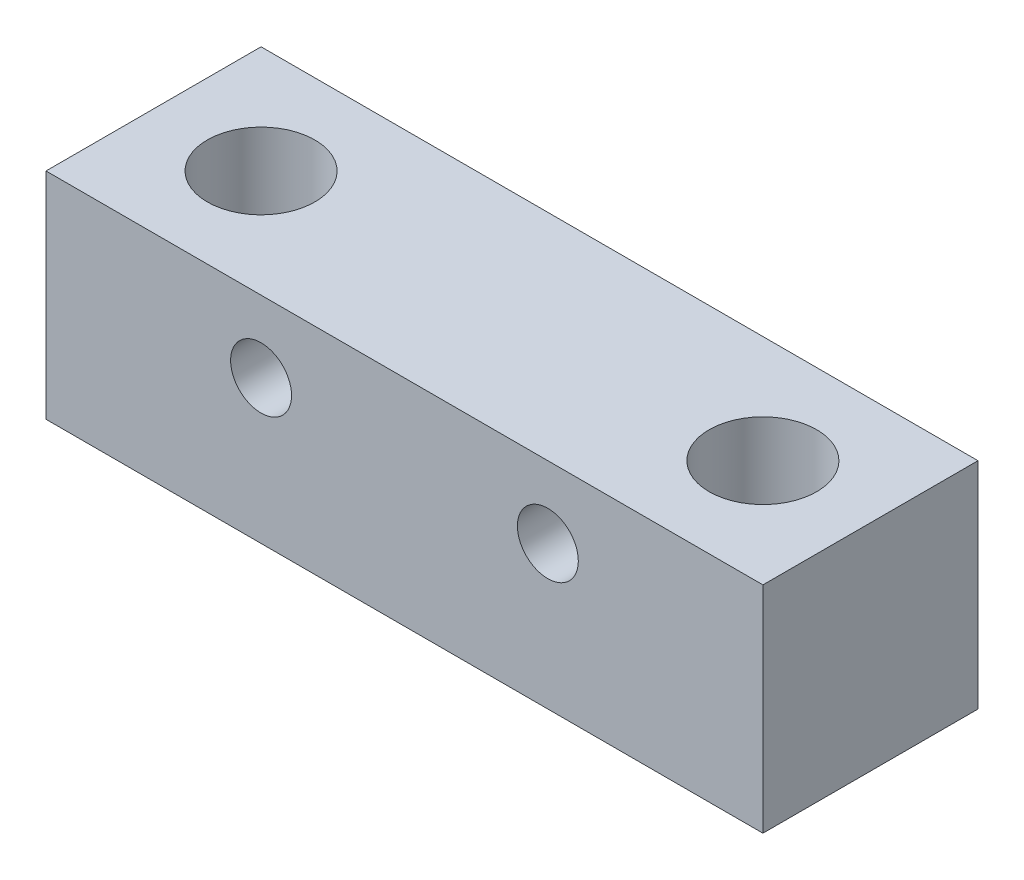
SolidWorks part; units mm, degrees
ref_plane "前视基准面" through (0, 0, 0) normal (0, 0, 1) x (1, 0, 0)
ref_plane "上视基准面" through (0, 0, 0) normal (0, 1, 0) x (1, 0, 0)
ref_plane "右视基准面" through (0, 0, 0) normal (1, 0, 0) x (0, 0, -1)
sketch "草图1" plane through (0, 0, 0) normal (0, 0, 1) x (1, 0, 0)
  line L1 (-50, 15) -> (50, 15)
  line L2 (-50, 15) -> (-50, -15)
  line L3 (-50, -15) -> (50, -15)
  line L4 (50, 15) -> (50, -15)
  line L5 (-50, 15) -> (50, -15) construction
  line L6 (-50, -15) -> (50, 15) construction
  point P0 (0, 0)
  dimension "D1" = 30
  dimension "D2" = 100
extrude "凸台-拉伸1" add sketch "草图1" along normal blind 30
hole_wizard "打孔尺寸(%根据)内六角圆柱头螺钉的类型1" positions "草图2" profile "草图3" counterbore size "M8" standard "GB" end condition through all
sketch "草图2" plane through (0, 15, 0) normal (0, 1, 0) x (1, 0, 0)
  line L0 (0, 0) -> (0, -40.624) construction
  line L2 (50, -15) -> (9.9649, -15) construction
  line L3 (50, -30) -> (50, 0) construction
  point P0 (-35, -15)
  point P2 (35, -15)
  dimension "D1" = 70
sketch "草图3" plane through (-35, 15, 15) normal (1, 0, 0) x (0, 0, 1)
  line L0 (0, 0) -> (0, 30)
  line L1 (0, 30) -> (4.5, 30)
  line L3 (4.5, 30) -> (4.5, 20)
  line L4 (4.5, 20) -> (7.5, 20)
  line L5 (7.5, 20) -> (7.5, 0)
  line L7 (7.5, 0) -> (0, 0)
  line L11 (0, -6.35) -> (0, 107.95) construction
  dimension "通孔孔直径" = 9
  dimension "通孔孔深度" = 30
  dimension "柱形沉头孔直径" = 15
  dimension "柱形沉头孔深度" = 20
hole_wizard "M10 螺纹孔1" positions "草图4" profile "草图5" tap size "M10" standard "GB" end condition through all
sketch "草图4" plane through (0, 0, 30) normal (0, 0, 1) x (1, 0, 0)
  line L0 (0, 41.3926) -> (0, 0) construction
  line L2 (-50, -15) -> (50, -15) construction
  point P0 (-20, 5)
  point P2 (20, 5)
  dimension "D1" = 40
  dimension "D2" = 20
sketch "草图5" plane through (-20, 5, 30) normal (1, 0, 0) x (0, -1, 0)
  line L0 (0, 0) -> (0, 30)
  line L1 (0, 30) -> (4.25, 30)
  line L2 (4.25, 30) -> (4.25, 0)
  line L5 (4.25, 0) -> (0, 0)
  line L11 (0, -6.35) -> (0, 107.95) construction
  dimension "通孔螺纹孔钻头直径" = 8.5
  dimension "通孔螺纹孔钻头深度" = 30
cosmetic thread "孔螺蚊线1" parameters "D2"=10
cosmetic thread "孔螺蚊线2" parameters "D2"=10
